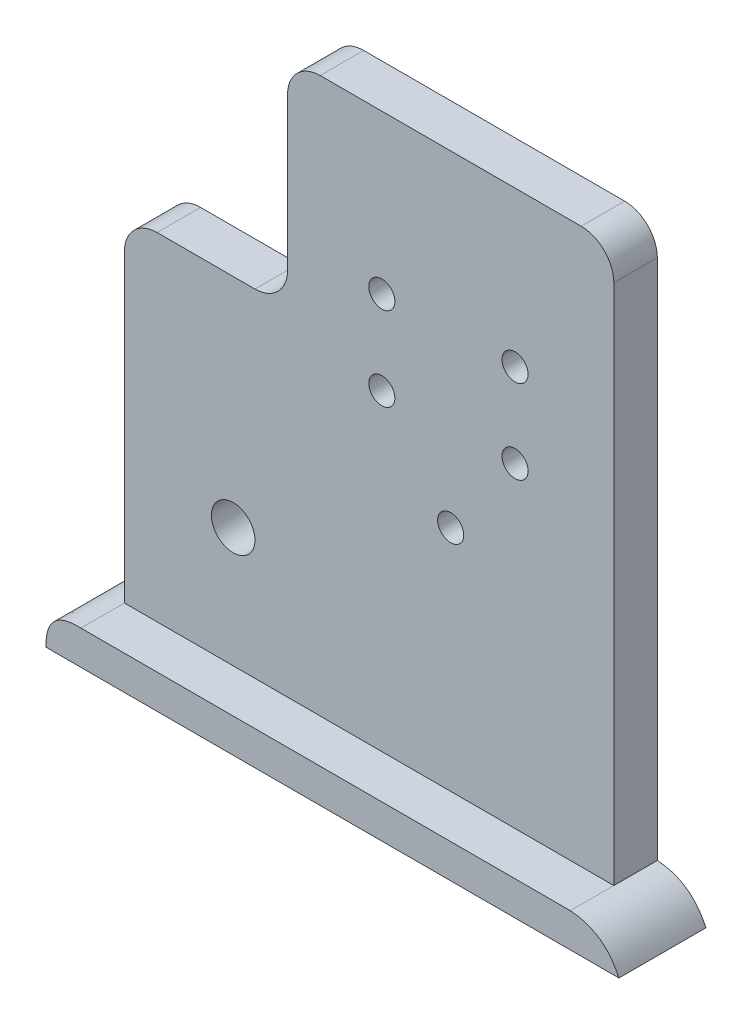
SolidWorks part; units mm, degrees
ref_plane "Front Plane" through (0, 0, 0) normal (0, 0, 1) x (1, 0, 0)
ref_plane "Top Plane" through (0, 0, 0) normal (0, 1, 0) x (1, 0, 0)
ref_plane "Right Plane" through (0, 0, 0) normal (1, 0, 0) x (0, 0, -1)
other "Configuration Table"
sketch "Sketch1" plane through (0, 0, 0) normal (0, 0, 1) x (1, 0, 0)
  line L1 (-300, 300) -> (300, 300)
  line L2 (-300, 300) -> (-300, -300)
  line L3 (-300, -300) -> (300, -300)
  line L4 (300, 300) -> (300, -300)
  line L5 (-300, 300) -> (300, -300) construction
  line L6 (-300, -300) -> (300, 300) construction
  point P0 (0, 0)
  dimension "D1" = 600
  dimension "D2" = 600
extrude "Boss-Extrude1" add sketch "Sketch1" along normal blind 40
sketch "Sketch2" plane through (0, 0, 40) normal (0, 0, 1) x (1, 0, 0)
  line L0 (-300, 300) -> (-300, -300) construction
  line L1 (-300, -300) -> (300, -300) construction
  circle A0 centre (-200, -100) radius 20
  dimension "D1" = 40
  dimension "D3" = 200
  dimension "D2" = 100
extrude "Cut-Extrude1" cut sketch "Sketch2" against normal blind 40
sketch "Sketch3" plane through (0, 0, 40) normal (0, 0, 1) x (1, 0, 0)
  line L0 (-300, 300) -> (-300, -300) construction
  circle A0 centre (0, 0) radius 12
  circle A1 centre (-200, -100) radius 20 construction
  dimension "D1" = 24
  dimension "D3" = 100
  dimension "D2" = 300
extrude "Cut-Extrude2" cut sketch "Sketch3" against normal blind 60
sketch "Sketch4" plane through (0, 0, 40) normal (0, 0, 1) x (1, 0, 0)
  circle A0 centre (-63.3353, 77.3863) radius 12
  circle A1 centre (59.1684, 80.617) radius 12
  circle A2 centre (0, 0) radius 12 construction
  dimension "D1" = 24
  dimension "D2" = 24
  dimension "D3" = 100
  dimension "D4" = 100
extrude "Cut-Extrude3" cut sketch "Sketch4" against normal blind 90
sketch "Sketch5" plane through (0, 0, 40) normal (0, 0, 1) x (1, 0, 0)
  line L0 (-300, -300) -> (300, -300) construction
  line L1 (300, 300) -> (150, 300)
  line L2 (300, 300) -> (300, -300)
  line L3 (300, -300) -> (150, -300)
  line L4 (150, 300) -> (150, -300)
  dimension "D1" = 150
extrude "Cut-Extrude4" cut sketch "Sketch5" against normal blind 100
sketch "Sketch6" plane through (0, 0, 40) normal (0, 0, 1) x (1, 0, 0)
  line L1 (-300, 300) -> (-150, 300)
  line L2 (-300, 300) -> (-300, 100)
  line L3 (-300, 100) -> (-150, 100)
  line L4 (-150, 300) -> (-150, 100)
  dimension "D1" = 150
  dimension "D2" = 200
extrude "Cut-Extrude5" cut sketch "Sketch6" against normal blind 100
sketch "Sketch7" plane through (0, 0, 40) normal (0, 0, 1) x (1, 0, 0)
  line L0 (150, 300) -> (150, -300) construction
  line L1 (-300, -300) -> (150, -300)
  line L2 (-300, -300) -> (-300, -210)
  line L3 (-300, -210) -> (150, -210)
  line L4 (150, -300) -> (150, -210)
  dimension "D1" = 90
extrude "Cut-Extrude6" cut sketch "Sketch7" against normal blind 100
sketch "Sketch9" plane through (0, 0, 40) normal (0, 0, 1) x (1, 0, 0)
  circle A0 centre (-63.3353, 154.3863) radius 12
  circle A1 centre (59.1684, 157.617) radius 12
  circle A2 centre (-63.3353, 77.3863) radius 12 construction
  circle A3 centre (59.1684, 80.617) radius 12 construction
  dimension "D1" = 24
  dimension "D2" = 24
  dimension "D3" = 77
  dimension "D4" = 77
extrude "Cut-Extrude7" cut sketch "Sketch9" against normal blind 50
fillet "Fillet1" radius 30 4 edges at (-300, 100, 20) (-150, 100, 20) (150, 300, 20) (-150, 300, 20)
sketch "Sketch10" plane through (0, 0, 0) normal (0, 0, -1) x (-1, 0, 0)
  line L0 (-150, -210) -> (300, -210)
  line L1 (-194.7025, -241.2649) -> (332.0537, -241.2649)
  spline S0 degree 2 poles (-150, -210) (-181.3128, -212.0592) (-194.7025, -241.2649) knots 0 0 0 1 1 1
  spline S1 degree 2 poles (300, -210) (333.1456, -208.5563) (332.0537, -241.2649) knots 0 0 0 1 1 1
extrude "Boss-Extrude2" add sketch "Sketch10" against normal blind 80
